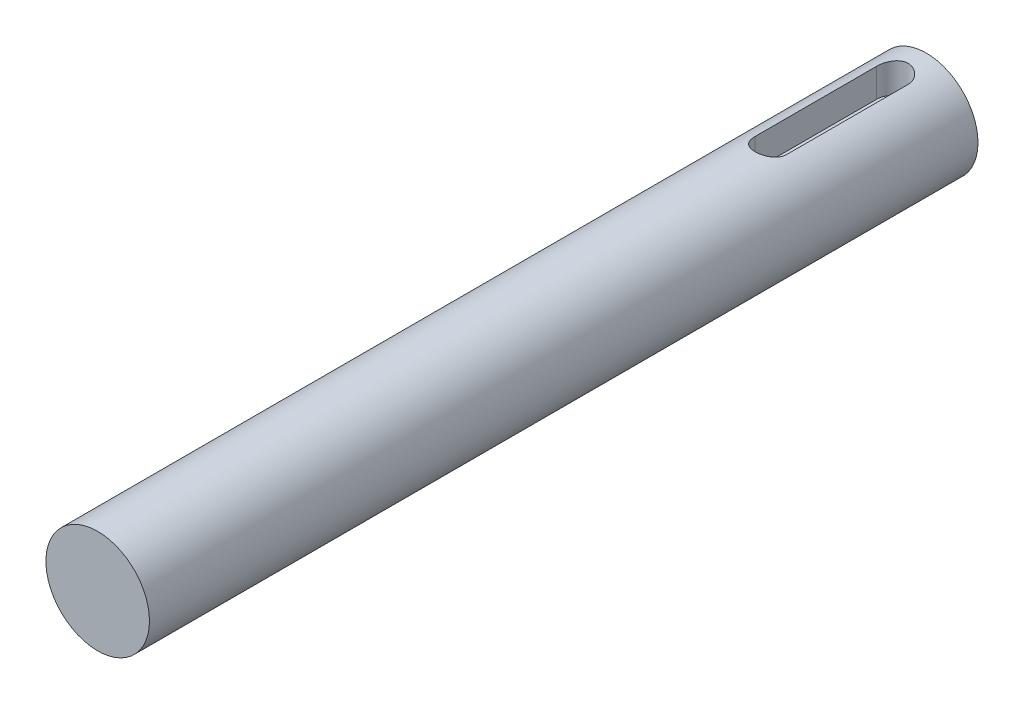
from build123d import *

# Parameters (mm, degrees)
SKETCH1_R           = 5
BOSS_EXTRUDE1_DEPTH = 80
CUT_EXTRUDE2_DEPTH  = 3


with BuildPart() as part:
    # Sketch1 → Boss-Extrude1 (new body)
    with BuildSketch(Plane.XY):
        Circle(SKETCH1_R)
    extrude(amount=BOSS_EXTRUDE1_DEPTH)

    # Sketch2 → Cut-Extrude2 (cut)
    with BuildSketch(Plane(origin=(0, 5, 0), x_dir=(1, 0, 0), z_dir=(0, 1, 0))):
        with BuildLine():
            Line((-1.519571935, -15), (-1.519571935, -3.259754454))
            ThreePointArc((-1.519571935, -3.259754454), (0, -1.740182518), (1.519571935, -3.259754454))
            Line((1.519571935, -3.259754454), (1.519571935, -15))
            ThreePointArc((1.519571935, -15), (0, -16.519571935), (-1.519571935, -15))
        make_face()
    extrude(amount=-CUT_EXTRUDE2_DEPTH, mode=Mode.SUBTRACT)


solid = part.part
